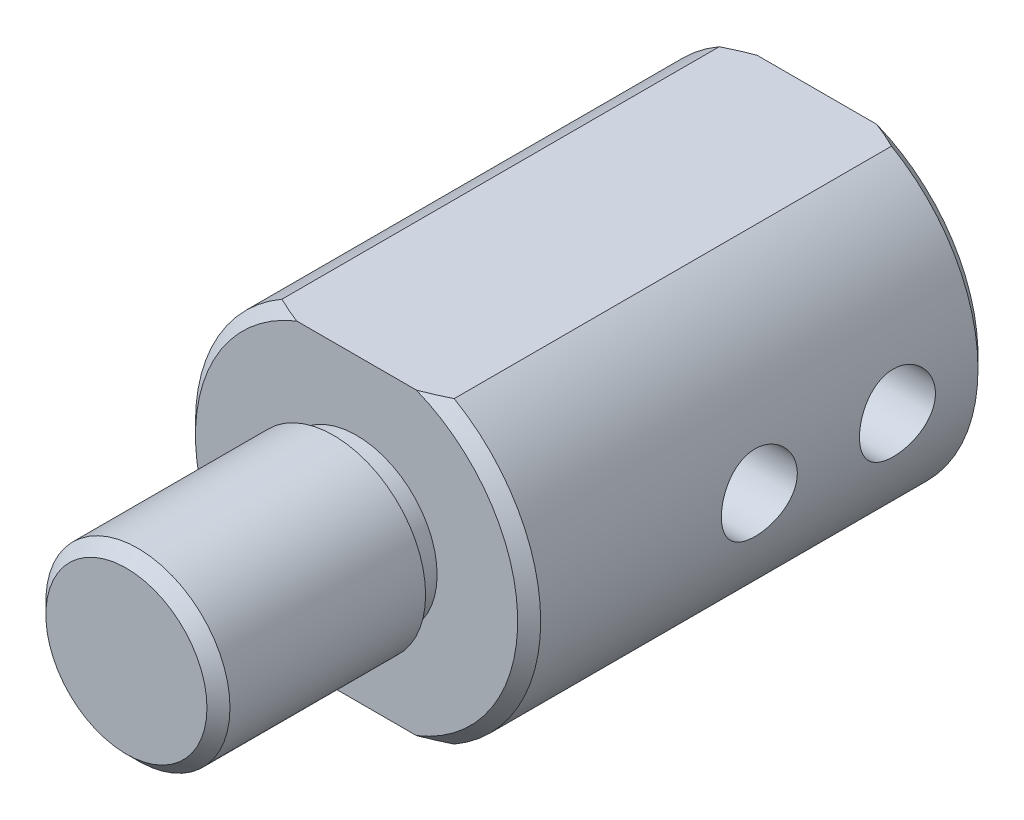
from build123d import *

# Parameters (mm, degrees)
SKETCH_1_R                  = 7.5
EXTRUDE_1_DEPTH             = 30
SKETCH_2_R                  = 8.226284638
SKETCH_2_R_2                = 4
CUT_EXTRUDE_1_DEPTH         = 10
SKETCH_3_R                  = 1.5
CUT_EXTRUDE_2_DEPTH         = 13
SKETCH_4_R                  = 4.479492859
SKETCH_4_R_2                = 3.5
CUT_EXTRUDE_3_DEPTH         = 1
CHAMFER_1_SIZE              = 0.5
SKETCH_6_W                  = 1.65
SKETCH_6_H                  = 7.5
HOLE_WIZARD_M4_1_AT_2_COUNT = 2
HOLE_WIZARD_M4_1_AT_2_PITCH = 6
SKETCH_7_W                  = 26.910087363
SKETCH_7_H                  = 4.855614415
SKETCH_7_W_2                = 23.143582724
SKETCH_7_H_2                = 3.131190604
CUT_EXTRUDE_4_DEPTH         = 5


with BuildPart() as part:
    # 草图1 → 凸台-拉伸1 (new body)
    with BuildSketch(Plane.XY):
        Circle(SKETCH_1_R)
    extrude(amount=EXTRUDE_1_DEPTH)

    # 草图2 → 切除-拉伸1 (cut)
    with BuildSketch(Plane.XY.offset(30)):
        Circle(SKETCH_2_R)
        Circle(SKETCH_2_R_2, mode=Mode.SUBTRACT)
    extrude(amount=-CUT_EXTRUDE_1_DEPTH, mode=Mode.SUBTRACT)

    # 草图3 → 切除-拉伸2 (cut)
    with BuildSketch(Plane(origin=(0, 0, 0), x_dir=(-1, 0, 0), z_dir=(0, 0, -1))):
        Circle(SKETCH_3_R)
    extrude(amount=-CUT_EXTRUDE_2_DEPTH, mode=Mode.SUBTRACT)

    # 草图4 → 切除-拉伸3 (cut)
    with BuildSketch(Plane.XY.offset(20)):
        Circle(SKETCH_4_R)
        Circle(SKETCH_4_R_2, mode=Mode.SUBTRACT)
    extrude(amount=CUT_EXTRUDE_3_DEPTH, mode=Mode.SUBTRACT)

    # 倒角1
    chamfer_1_edges = [part.edges().sort_by_distance(p)[0] for p in [
        (-7.5, 0, 0),
        (-7.5, 0, 20),
        (-4, 0, 30),
    ]]
    chamfer(chamfer_1_edges, length=CHAMFER_1_SIZE)

    # 草图6 → M4 螺纹孔1 (revolve, cut)
    with BuildSketch(Plane(origin=(0, 0, 4), x_dir=(0, 0, 1), z_dir=(0, 1, 0))):
        with Locations((0.825, 3.75)):
            Rectangle(SKETCH_6_W, SKETCH_6_H)
    hole_wizard_m4_1 = revolve(axis=Axis((-6.35, 0, 4), (1, 0, 0)), mode=Mode.SUBTRACT)

    # M4 螺纹孔1 at 2: M4 螺纹孔1 ×2
    with Locations(*[(0, 0, i * HOLE_WIZARD_M4_1_AT_2_PITCH) for i in range(1, HOLE_WIZARD_M4_1_AT_2_COUNT)]):
        add(hole_wizard_m4_1, mode=Mode.SUBTRACT)

    # 草图7 → 切除-拉伸4 (cut, symmetric)
    with BuildSketch(Plane(origin=(0, 0, 0), x_dir=(0, 0, -1), z_dir=(1, 0, 0))):
        with Locations((-11.641911526, 8.927807208)):
            Rectangle(SKETCH_7_W, SKETCH_7_H)
        with Locations((-10.167075372, -8.065595302)):
            Rectangle(SKETCH_7_W_2, SKETCH_7_H_2)
    extrude(amount=CUT_EXTRUDE_4_DEPTH, both=True, mode=Mode.SUBTRACT)


solid = part.part
